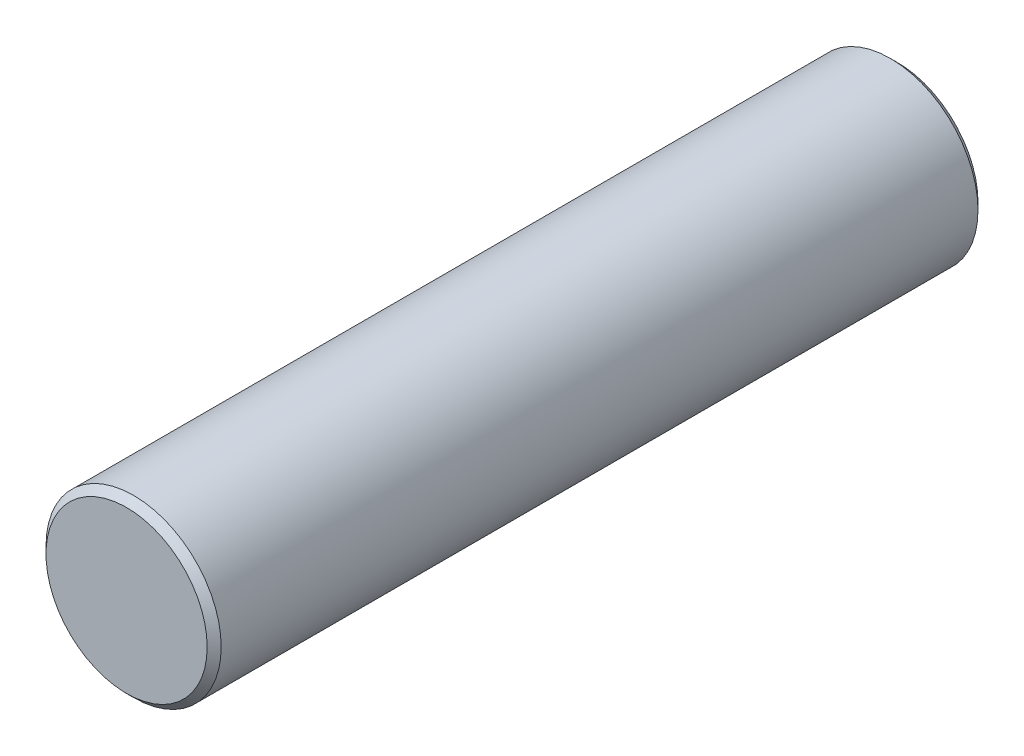
from build123d import *

# Parameters (mm, degrees)
SKETCH1_R           = 25
BOSS_EXTRUDE1_DEPTH = 220
CHAMFER1_SIZE       = 2


with BuildPart() as part:
    # Sketch1 → Boss-Extrude1 (new body)
    with BuildSketch(Plane.XY):
        Circle(SKETCH1_R)
    extrude(amount=BOSS_EXTRUDE1_DEPTH)

    # Chamfer1
    chamfer1_edges = [part.edges().sort_by_distance(p)[0] for p in [
        (-25, 0, 0),
        (-25, 0, 220),
    ]]
    chamfer(chamfer1_edges, length=CHAMFER1_SIZE)


solid = part.part
